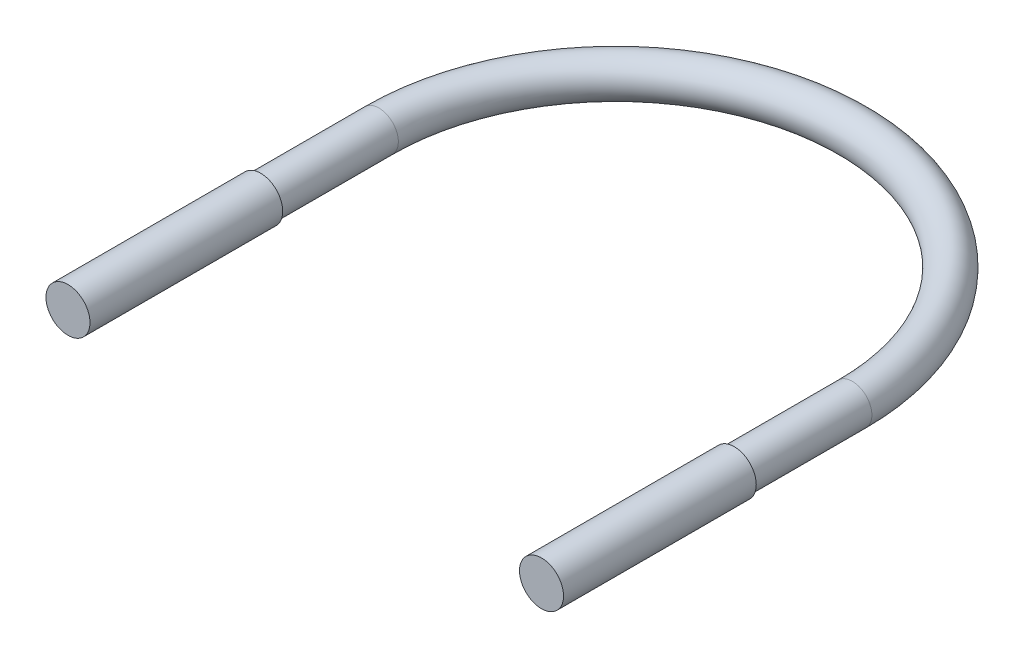
SolidWorks part; units mm, degrees
material "SUS 304"
ref_plane "前视基准面" through (0, 0, 0) normal (0, 0, 1) x (1, 0, 0)
ref_plane "上视基准面" through (0, 0, 0) normal (0, 1, 0) x (1, 0, 0)
ref_plane "右视基准面" through (0, 0, 0) normal (1, 0, 0) x (0, 0, -1)
sketch "草图1" plane through (0, 0, 0) normal (0, 0, 1) x (1, 0, 0)
  circle A0 centre (0, 0) radius 3.55
  dimension "D1" = 7.1
sketch "草图2" plane through (0, 0, 0) normal (0, 1, 0) x (1, 0, 0)
  line L0 (0, 56.45) -> (0, 0)
  line L1 (86, 56.45) -> (86, 0)
  arc A0 (86, 56.45) -> (0, 56.45) centre (43, 56.45) ccw
  dimension "D1" = 86
  dimension "D2" = 43
  dimension "D3" = 99.45
sweep "扫描1" add profiles "草图1" path "草图2"
sketch "草图3" plane through (0, 0, 0) normal (0, 0, 1) x (1, 0, 0)
  circle A0 centre (0, 0) radius 4
  circle A1 centre (86, 0) radius 4
  dimension "D1" = 8
  dimension "D2" = 8
extrude "凸台-拉伸1" add sketch "草图3" against normal blind 35
cosmetic thread "装饰螺纹线1" parameters "D2"=7
cosmetic thread "装饰螺纹线2" parameters "D2"=7
